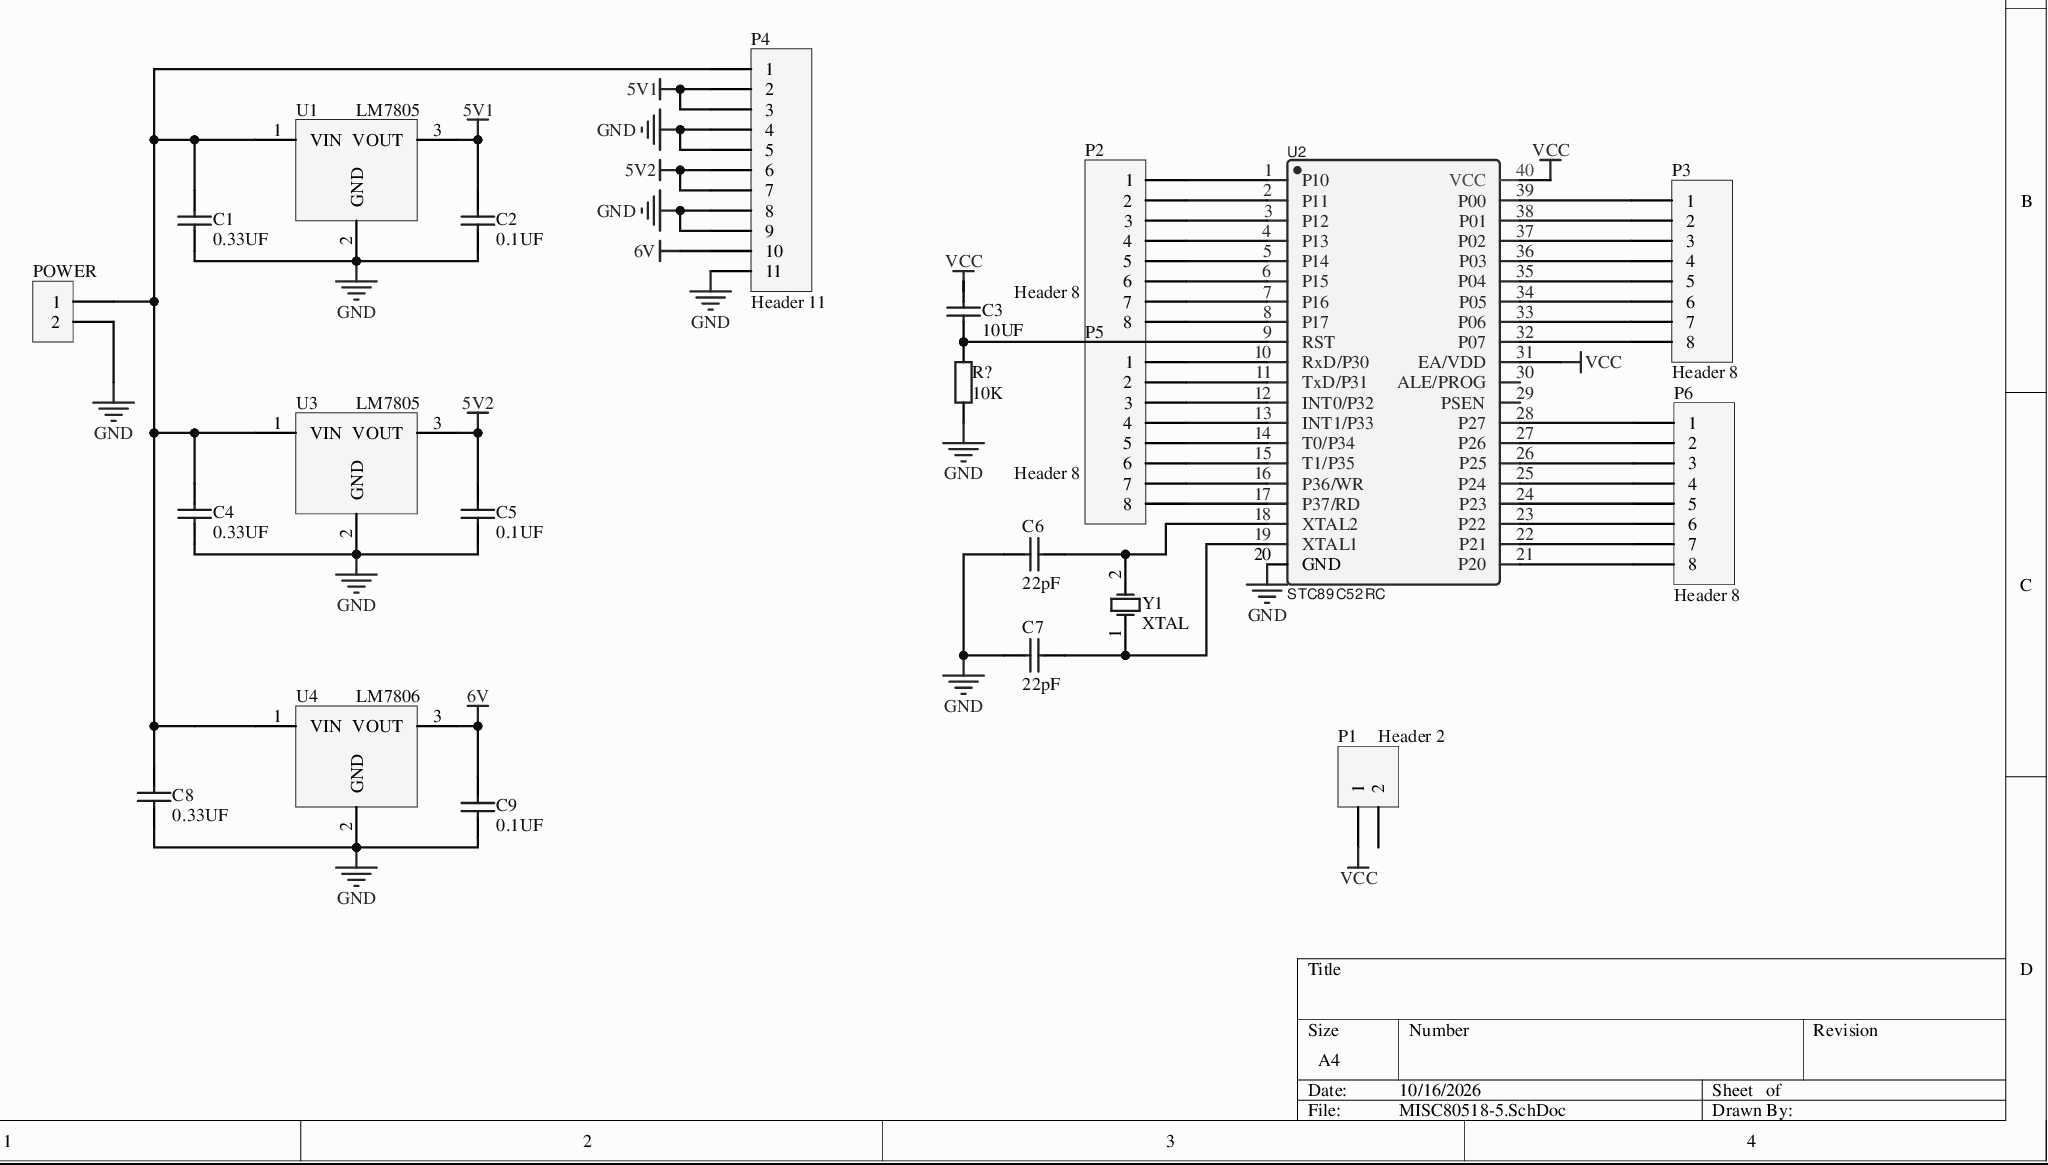
[diagram p0: MISC80518-5.SchDoc]
# Altium project MISC80518-2.PrjPcb
1 sheet, 22 parts. Net scope: global (net labels, ports and power ports of the same name join across sheets).
Board file: MISC80518.PcbDoc

## Sheet MISC80518-5.SchDoc
size A4

### Parts
C1  0.33UF  [RAD-0.3]
C2  0.1UF  [RAD-0.3]
C3  10UF  [RAD-0.3]
C4  0.33UF  [RAD-0.3]
C5  0.1UF  [RAD-0.3]
C6  22pF  [RAD-0.3]
C7  22pF  [RAD-0.3]
C8  0.33UF  [RAD-0.3]
C9  0.1UF  [RAD-0.3]
P1  Header 2  [HDR1X2]
P2  Header 8  [HDR1X8]
P3  Header 8  [HDR1X8]
P4  Header 11  [HDR1X11]
P5  Header 8  [HDR1X8]
P6  Header 8  [HDR1X8]
POWER  Terminal block  [VH3.96-2A]  (value not drawn)
R?  10K  [AXIAL-0.4]
U1  LM7805  [TO220A]
U2  STC89C52RC  [STC89C52RC]
U3  LM7805  [TO220A]
U4  LM7806  [TO220A]
Y1  XTAL  [R38]

### Nets
5V1: C2.1 P4.2 P4.3 U1.3(VOUT)
5V2: C5.1 P4.6 P4.7 U3.3(VOUT)
6V: C9.1 P4.10 U4.3(VOUT)
GND: C1.2 C2.2 C4.2 C5.2 C6.2 C7.2 C8.2 C9.2 P4.4 P4.5 P4.8 P4.9 P4.11 POWER.2 R?.1 U1.2(GND) U2.20(GND) U3.2(GND) U4.2(GND)
VCC: C3.1 P1.1 U2.31(EA/VDD) U2.40(VCC)
NetC1_1: C1.1 C4.1 C8.1 P4.1 POWER.1 U1.1(VIN) U3.1(VIN) U4.1(VIN)
NetC3_2: C3.2 R?.2 U2.9(RST)
NetC6_1: C6.1 U2.18(XTAL2) Y1.2(OSC2)
NetC7_1: C7.1 U2.19(XTAL1) Y1.1(OSC1)
NetP2_1: P2.1 U2.1(P10)
NetP2_2: P2.2 U2.2(P11)
NetP2_3: P2.3 U2.3(P12)
NetP2_4: P2.4 U2.4(P13)
NetP2_5: P2.5 U2.5(P14)
NetP2_6: P2.6 U2.6(P15)
NetP2_7: P2.7 U2.7(P16)
NetP2_8: P2.8 U2.8(P17)
NetP3_1: P3.1 U2.39(P00)
NetP3_2: P3.2 U2.38(P01)
NetP3_3: P3.3 U2.37(P02)
NetP3_4: P3.4 U2.36(P03)
NetP3_5: P3.5 U2.35(P04)
NetP3_6: P3.6 U2.34(P05)
NetP3_7: P3.7 U2.33(P06)
NetP3_8: P3.8 U2.32(P07)
NetP5_1: P5.1 U2.10(RxD/P30)
NetP5_2: P5.2 U2.11(TxD/P31)
NetP5_3: P5.3 U2.12(INT0/P32)
NetP5_4: P5.4 U2.13(INT1/P33)
NetP5_5: P5.5 U2.14(T0/P34)
NetP5_6: P5.6 U2.15(T1/P35)
NetP5_7: P5.7 U2.16(P36/WR)
NetP5_8: P5.8 U2.17(P37/RD)
NetP6_1: P6.1 U2.28(P27)
NetP6_2: P6.2 U2.27(P26)
NetP6_3: P6.3 U2.26(P25)
NetP6_4: P6.4 U2.25(P24)
NetP6_5: P6.5 U2.24(P23)
NetP6_6: P6.6 U2.23(P22)
NetP6_7: P6.7 U2.22(P21)
NetP6_8: P6.8 U2.21(P20)

Not connected (* = marked no-connect by the designer): P1 2; U2 29(PSEN) 30(ALE/PROG)

### Library data of the parts
C1-C9 = Cap: Capacitor; Value: 100pF; Published: 8-Jun-2000; LatestRevisionDate: 17-Jul-2002; LatestRevisionNote: Re-released for DXP Platform.; PackageReference: RAD-0.3; PackageDescription: Radial Cap, Thru-Hole; 2 Leads; 0.3 in Pin Spacing; Publisher: Altium Limited
P1 = Header 2: Header, 2-Pin; LatestRevisionDate: 17-Jul-2002; LatestRevisionNote: Re-released for DXP Platform.; Publisher: Altium Limited
P2 P3 P5 P6 = Header 8: Header, 8-Pin; LatestRevisionDate: 17-Jul-2002; LatestRevisionNote: Re-released for DXP Platform.; Publisher: Altium Limited
P4 = Header 11: Header, 11-Pin; LatestRevisionDate: 17-Jul-2002; LatestRevisionNote: Re-released for DXP Platform.; Publisher: Altium Limited
POWER = VH2
R? = Res2: Resistor; Value: 1K; Published: 8-Jun-2000; LatestRevisionDate: 17-Jul-2002; LatestRevisionNote: Re-released for DXP Platform.; PackageReference: AXIAL-0.4; PackageDescription: Axial Device, Thru-Hole; 2 Leads; 0.4 in Pin Spacing; Publisher: Altium Limited
U4 = LM7805
Y1 = XTAL: Crystal Oscillator; Published: 8-Jun-2000; LatestRevisionDate: 17-Jul-2002; LatestRevisionNote: Re-released for DXP Platform.; PackageReference: R38; PackageDescription: Crystal, Thru-Hole; 2 Leads; Body 3.1 x 8.2 mm (Dia.xH); Publisher: Altium Limited